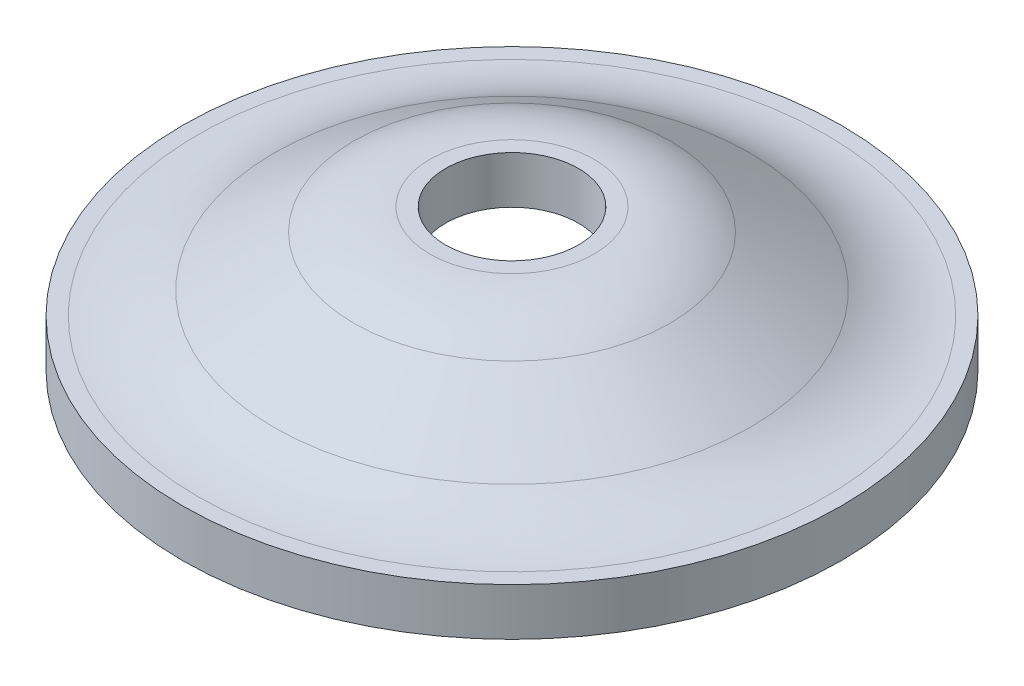
SolidWorks part; units mm, degrees
material "成品"
ref_plane "Front Plane" through (0, 0, 0) normal (0, 0, 1) x (1, 0, 0)
ref_plane "Top Plane" through (0, 0, 0) normal (0, 1, 0) x (1, 0, 0)
ref_plane "Right Plane" through (0, 0, 0) normal (1, 0, 0) x (0, 0, -1)
sketch "Sketch1" plane through (0, 0, 0) normal (0, 0, 1) x (1, 0, 0)
  line L0 (0, 0) -> (0, -50.7267) construction
  line L7 (-2.8, 0) -> (-3.4635, 0)
  line L9 (-13.2365, -3.98) -> (-13.9, -3.98)
  line L10 (-13.9, -3.98) -> (-13.9, -5.98)
  line L11 (-13.9, -5.98) -> (-13.2365, -5.98)
  line L13 (-3.4635, -2) -> (-2.8, -2)
  line L14 (-2.8, -2) -> (-2.8, 0)
  line L18 (-6.6681, -2.9274) -> (-10.0319, -5.0526)
  line L19 (-10.0319, -3.0526) -> (-6.6681, -0.9274)
  line L20 (-8.35, -1.99) -> (-8.35, -3.99) construction
  arc A0 (-3.4635, 0) -> (-6.6681, -0.9274) centre (-3.4635, -6) ccw
  arc A1 (-3.4635, -2) -> (-6.6681, -2.9274) centre (-3.4635, -8) ccw
  arc A2 (-10.0319, -5.0526) -> (-13.2365, -5.98) centre (-13.2365, 0.02) cw
  arc A3 (-10.0319, -3.0526) -> (-13.2365, -3.98) centre (-13.2365, 2.02) cw
  point P16 (-5.2, -2)
  point P20 (-11.5, -5.98)
  dimension "D6" = 2
  dimension "D7" = 2.4
  dimension "D9" = 6
  dimension "D1" = 5.98
  dimension "D2" = 2
  dimension "D3" = 27.8
  dimension "D4" = 5.6
  dimension "D5" = 2
  dimension "D8" = 2.4
revolve "Revolve1" add sketch "Sketch1" angle 360 about L0
